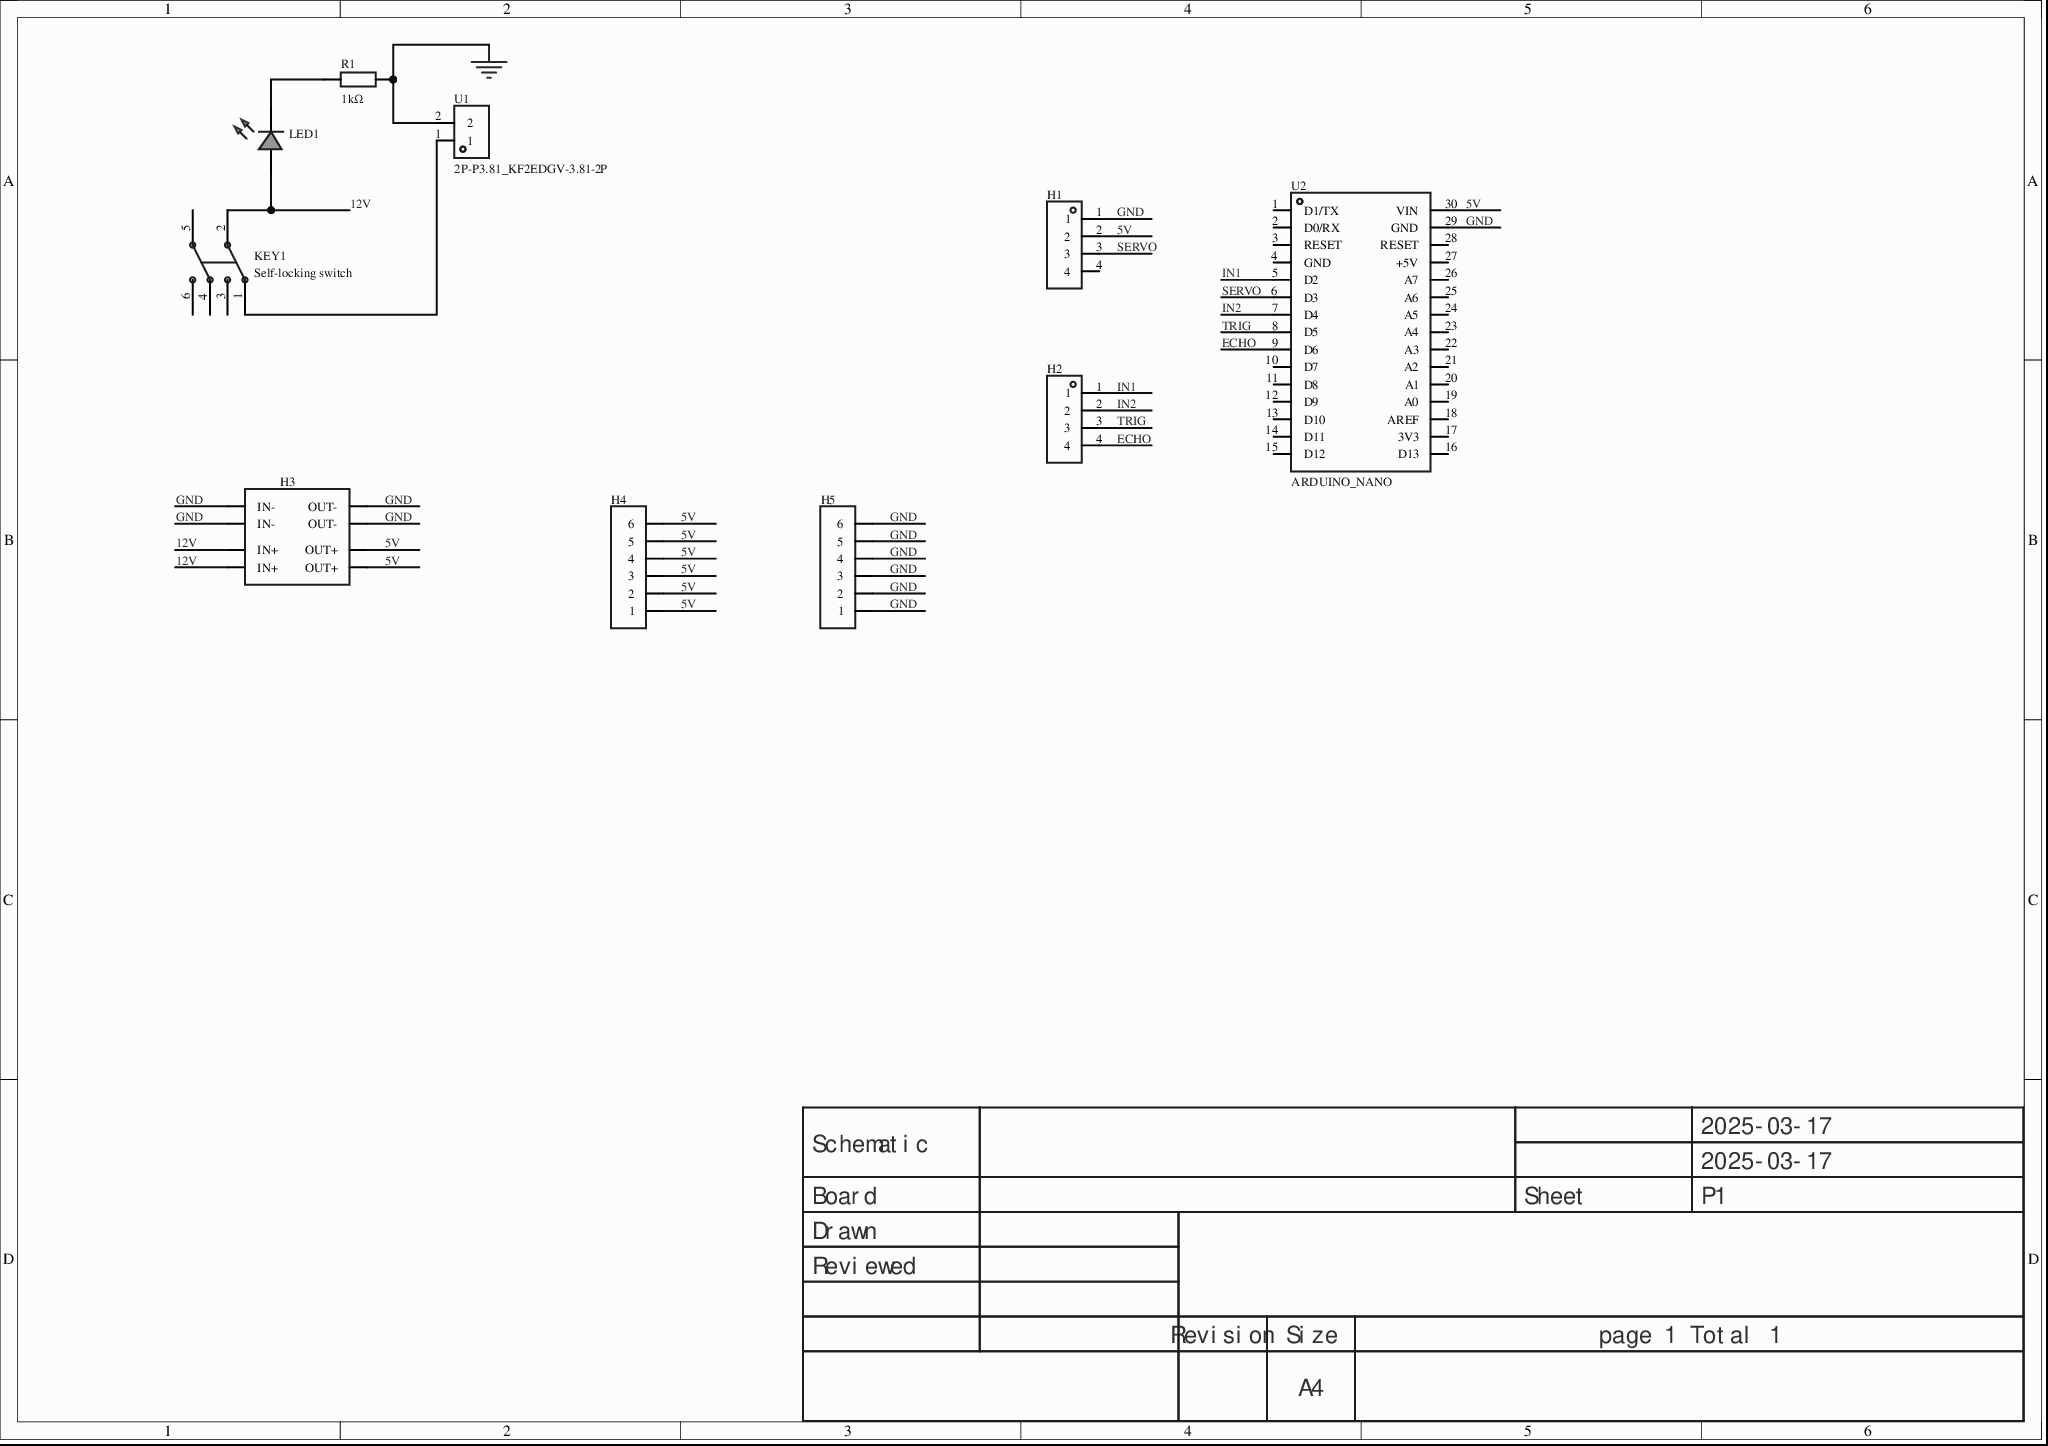
[diagram p0: MISC49855-3.schdoc]
# Altium project MISC49855-2.PrjPcb
1 sheet, 10 parts. Net scope: global (net labels, ports and power ports of the same name join across sheets).
Board file: MISC49855.pcbdoc

## Sheet MISC49855-3.schdoc
size 297 x 209 mm; Version: V1.0; @Project Name: MISC49855; @Page Count: 1; @Update Date: 2025-03-17; @Create Date: 2025-03-17; @Schematic Name: MISC49855; @Page No: 1; @Create Time: 21:11:00; @Update Time: 21:22:56; @Board Name: MISC49855

### Parts
H1  (no value)  [HDR-TH_4P-P2.54-V-M]
H2  (no value)  [HDR-TH_4P-P2.54-V-M]
H3  (no value)  [HDR-TH_8P-P2.54-V-M]
H4  (no value)  [HDR-TH_6P-P2.54-V-M-1]
H5  (no value)  [HDR-TH_6P-P2.54-V-M-1]
KEY1  Self-locking switch  [SW-TH_6P-L8.5-W8.5-P2.54]
LED1  (no value)  [LED_TH-3mm]
R1  1kΩ  [Res_1/4W]
U1  2P-P3.81_KF2EDGV-3.81-2P  [CONN-TH_2P-P3.81_KF2EDGV-3.81-2P]
U2  ARDUINO_NANO  [COMM-TH_ARDUINO_NANO]

### Nets
GND: H1.1 H3.1(IN-) H3.2(IN-) H3.5(OUT-) H3.6(OUT-) H5.1 H5.2 H5.3 H5.4 H5.5 H5.6 R1.2 U1.2 U2.29(GND)
5V: H1.2 H3.7(OUT+) H3.8(OUT+) H4.1 H4.2 H4.3 H4.4 H4.5 H4.6 U2.30(VIN)
12V: H3.3(IN+) H3.4(IN+) KEY1.2 LED1.1(C)
ECHO: H2.4 U2.9(D6)
IN1: H2.1 U2.5(D2)
IN2: H2.2 U2.7(D4)
SERVO: H1.3 U2.6(D3)
TRIG: H2.3 U2.8(D5)
NetKEY1_1: KEY1.1 U1.1
NetLED1_2: LED1.2(A) R1.1

Not connected (* = marked no-connect by the designer): H1 4*; KEY1 3 4 5 6; U2 1(D1/TX)* 2(D0/RX)* 3(RESET)* 4(GND)* 10(D7)* 11(D8)* 12(D9)* 13(D10)* 14(D11)* 15(D12)* 16(D13)* 17(3V3)* 18(AREF)* 19(A0)* 20(A1)* 21(A2)* 22(A3)* 23(A4)* 24(A5)* 25(A6)* 26(A7)* 27(+5V)* 28(RESET)*

### Notes on the sheet
- 2025-03-17
- Schematic
- Board
- Sheet
- P1
- Drawn
- Reviewed
- Revision
- Size
- A4
- page 1 Total 1

### Library data of the parts
H1 H2 = HDR-M_2.54_1x4P: Symbol: PZ254V-11-04P; ConvertToPcb: yes; ModelId: 112f4d05e8d64e99ab9a333894bea4f9; ModelName: HDR-TH_4P-P2.54-M-LI-1X4P; ModelTransform: 399.999,104.7242,0,0,0,0,0,0,-118.11; Device: HDR-M_2.54_1x4P; AddInBom: yes; SupplierPart: C492403; Supplier Footprint: 插件; FootprintName: HDR-TH_4P-P2.54-V-M
H3 = HDR-M_2.54_1x8P: Symbol: Header-Male-2.54_1x8; ConvertToPcb: yes; ModelId: f5b96e27511e49e38545e53df2320202; ModelTransform: 807.87244,98.425,0,0,0,0,0,0,-118.11; Device: HDR-M_2.54_1x8P; AddInBom: yes; SupplierPart: C124381; Supplier Footprint: 插件; FootprintName: HDR-TH_8P-P2.54-V-M; ModelName: HDR-TH_8P-P2.54-V-M
H4 H5 = HDR-M_2.54_1x6P: Symbol: Header-Male-2.54_1x6; ConvertToPcb: yes; ModelId: 60739dffc9b04830a286435b0fefbd4a; ModelName: HDR2.54-M-LI-1X6P; ModelTransform: 599.999,100,0,0,0,0,0,0,-118.11; Device: HDR-M_2.54_1x6P; AddInBom: yes; SupplierPart: C37208; Supplier Footprint: 插件; FootprintName: HDR-TH_6P-P2.54-V-M-1
KEY1 = 无自锁开关 8.5×8.5 无声: 6脚，8.5×8.5; Manufacturer Part: 自锁开关; Symbol: No self-locking switch 8.5×8.5 silent; AddInBom: yes; ModelId: 4c72b3966b92446eb355e1bd0fb4f880; ModelTransform: 342.519,334.645,0,180,0,0,0,0,-137.795; Description: 6 pins, 8.5×8.5; Device: No self-locking switch 8.5×8.5 silent; LCSC Part Name: 无自锁开关 8.5×8.5  无声; SupplierPart: C26228; Supplier Footprint: 插件; JLCPCB Part Class: Extended library; Supplier: LCSC; ConvertToPcb: yes; FootprintName: SW-TH_6P-L8.5-W8.5-P2.54; ModelName: SW-TH_6P-L8.5-W8.5-P2.54
LED1 = LED_TH-G_3mm: ConvertToPcb: yes; ModelId: a497c992633541038a38947cdc58012f; ModelName: LED-TH-3mm_R; ModelTransform: 141.274,153.327,0,0,0,0,-5.984,0,-137.795; Device: LED_TH-G_3mm; AddInBom: yes; SymbolName: LED_TH-G; FootprintName: LED_TH-3mm; Supplier Footprint: 插件
R1 = Res_AXIAL-1/4W: AddInBom: yes; SymbolName: Resistor; ModelId: 463263665006444ab7a47bd11b0cf956; ModelName: RES-TH_BD2.4-L6.3-P10.30-D0.6; ModelTransform: 427.165,94.32816,0,0,0,0,0,0,-196.85; Value: 1kΩ; Device: Res_AXIAL-1/4W; Supplier Footprint: 轴向引线; ConvertToPcb: yes; FootprintName: Res_1/4W
U1 = 2P-P3.81_KF2EDGV-3.81-2P: AddInBom: yes; ModelId: d0e460b57cc144faafea3ccd6ba14e93; ModelTransform: 331.4954,283.50337,0,0,0,0,0,-23.622,-137.795; Symbol: 2P-P3.81_KF2EDGV-3.81-2P; Device: 2P-P3.81_KF2EDGV-3.81-2P; LCSC Part Name: 2P-P3.81_KF2EDGV-3.81-2P; SupplierPart: C9900017459; ManufacturerPart: 2P-P3.81_KF2EDGV-3.81-2P; Supplier Footprint: CONN-TH_2P-P3.81_KF2EDGV-3.81-2P; JLCPCB Part Class: Extended library; Supplier: LCSC; ConvertToPcb: yes; FootprintName: CONN-TH_2P-P3.81_KF2EDGV-3.81-2P; ModelName: CONN-TH_2P-P3.81_KF2EDGV-3.81-2P
U2 = ARDUINO_NANO: AddInBom: yes; ModelId: 569460a3ee974a868db0f4d8fd87e38b; ModelTransform: 699.9986,1784.14604,0,270,0,0,-42.323,0,-137.795; Symbol: ARDUINO_NANO; Device: ARDUINO_NANO; LCSC Part Name: ARDUINO_NANO; SupplierPart: C9900017879; ManufacturerPart: ARDUINO_NANO; Supplier Footprint: 插件; JLCPCB Part Class: Extended library; Supplier: LCSC; ConvertToPcb: yes; FootprintName: COMM-TH_ARDUINO_NANO; ModelName: ARDUINO_NANO